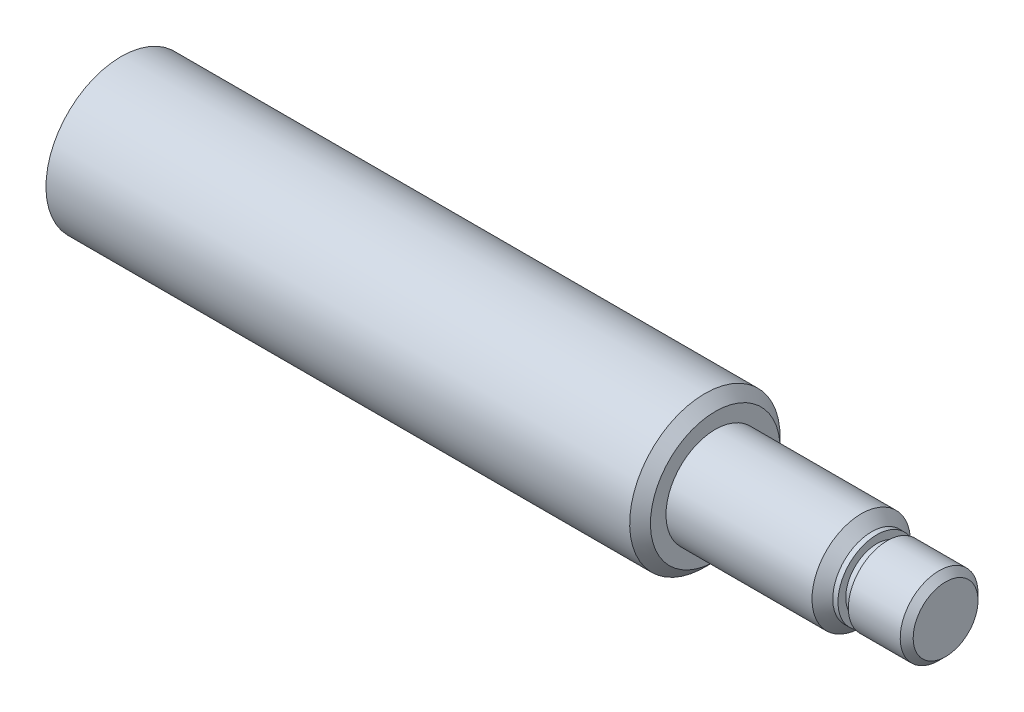
SolidWorks part; units mm, degrees
ref_plane "Front Plane" through (0, 0, 0) normal (0, 0, 1) x (1, 0, 0)
ref_plane "Top Plane" through (0, 0, 0) normal (0, 1, 0) x (1, 0, 0)
ref_plane "Right Plane" through (0, 0, 0) normal (1, 0, 0) x (0, 0, -1)
other "Configuration Table"
sketch "Sketch1" plane through (0, 0, 0) normal (0, 0, 1) x (1, 0, 0)
  line L0 (838.3726, 0) -> (476.0263, 0) construction
  line L1 (828.3726, 15) -> (808.3726, 15)
  line L2 (804.3726, 15) -> (802.3726, 15)
  line L3 (808.3726, 12) -> (804.3726, 12)
  line L4 (738.0726, 29) -> (684.5826, 29)
  line L5 (684.5826, 29) -> (666.5826, 29)
  line L6 (666.5826, 29) -> (513.0226, 29)
  line L7 (830.8726, 12.5) -> (830.8726, 0)
  line L8 (798.3726, 19) -> (802.3726, 15)
  line L9 (828.3726, 15) -> (830.8726, 12.5)
  line L10 (738.0726, 29) -> (742.0726, 25)
  line L11 (742.0726, 25) -> (742.0726, 19)
  line L12 (798.3726, 19) -> (742.0726, 19)
  line L13 (808.3726, 15) -> (808.3726, 12)
  line L14 (804.3726, 15) -> (804.3726, 12)
  line L15 (513.0226, 29) -> (513.0226, 0)
  line L16 (513.0226, 0) -> (830.8726, 0)
revolve "Revolve1" add sketch "Sketch1" angle 360 about L0
